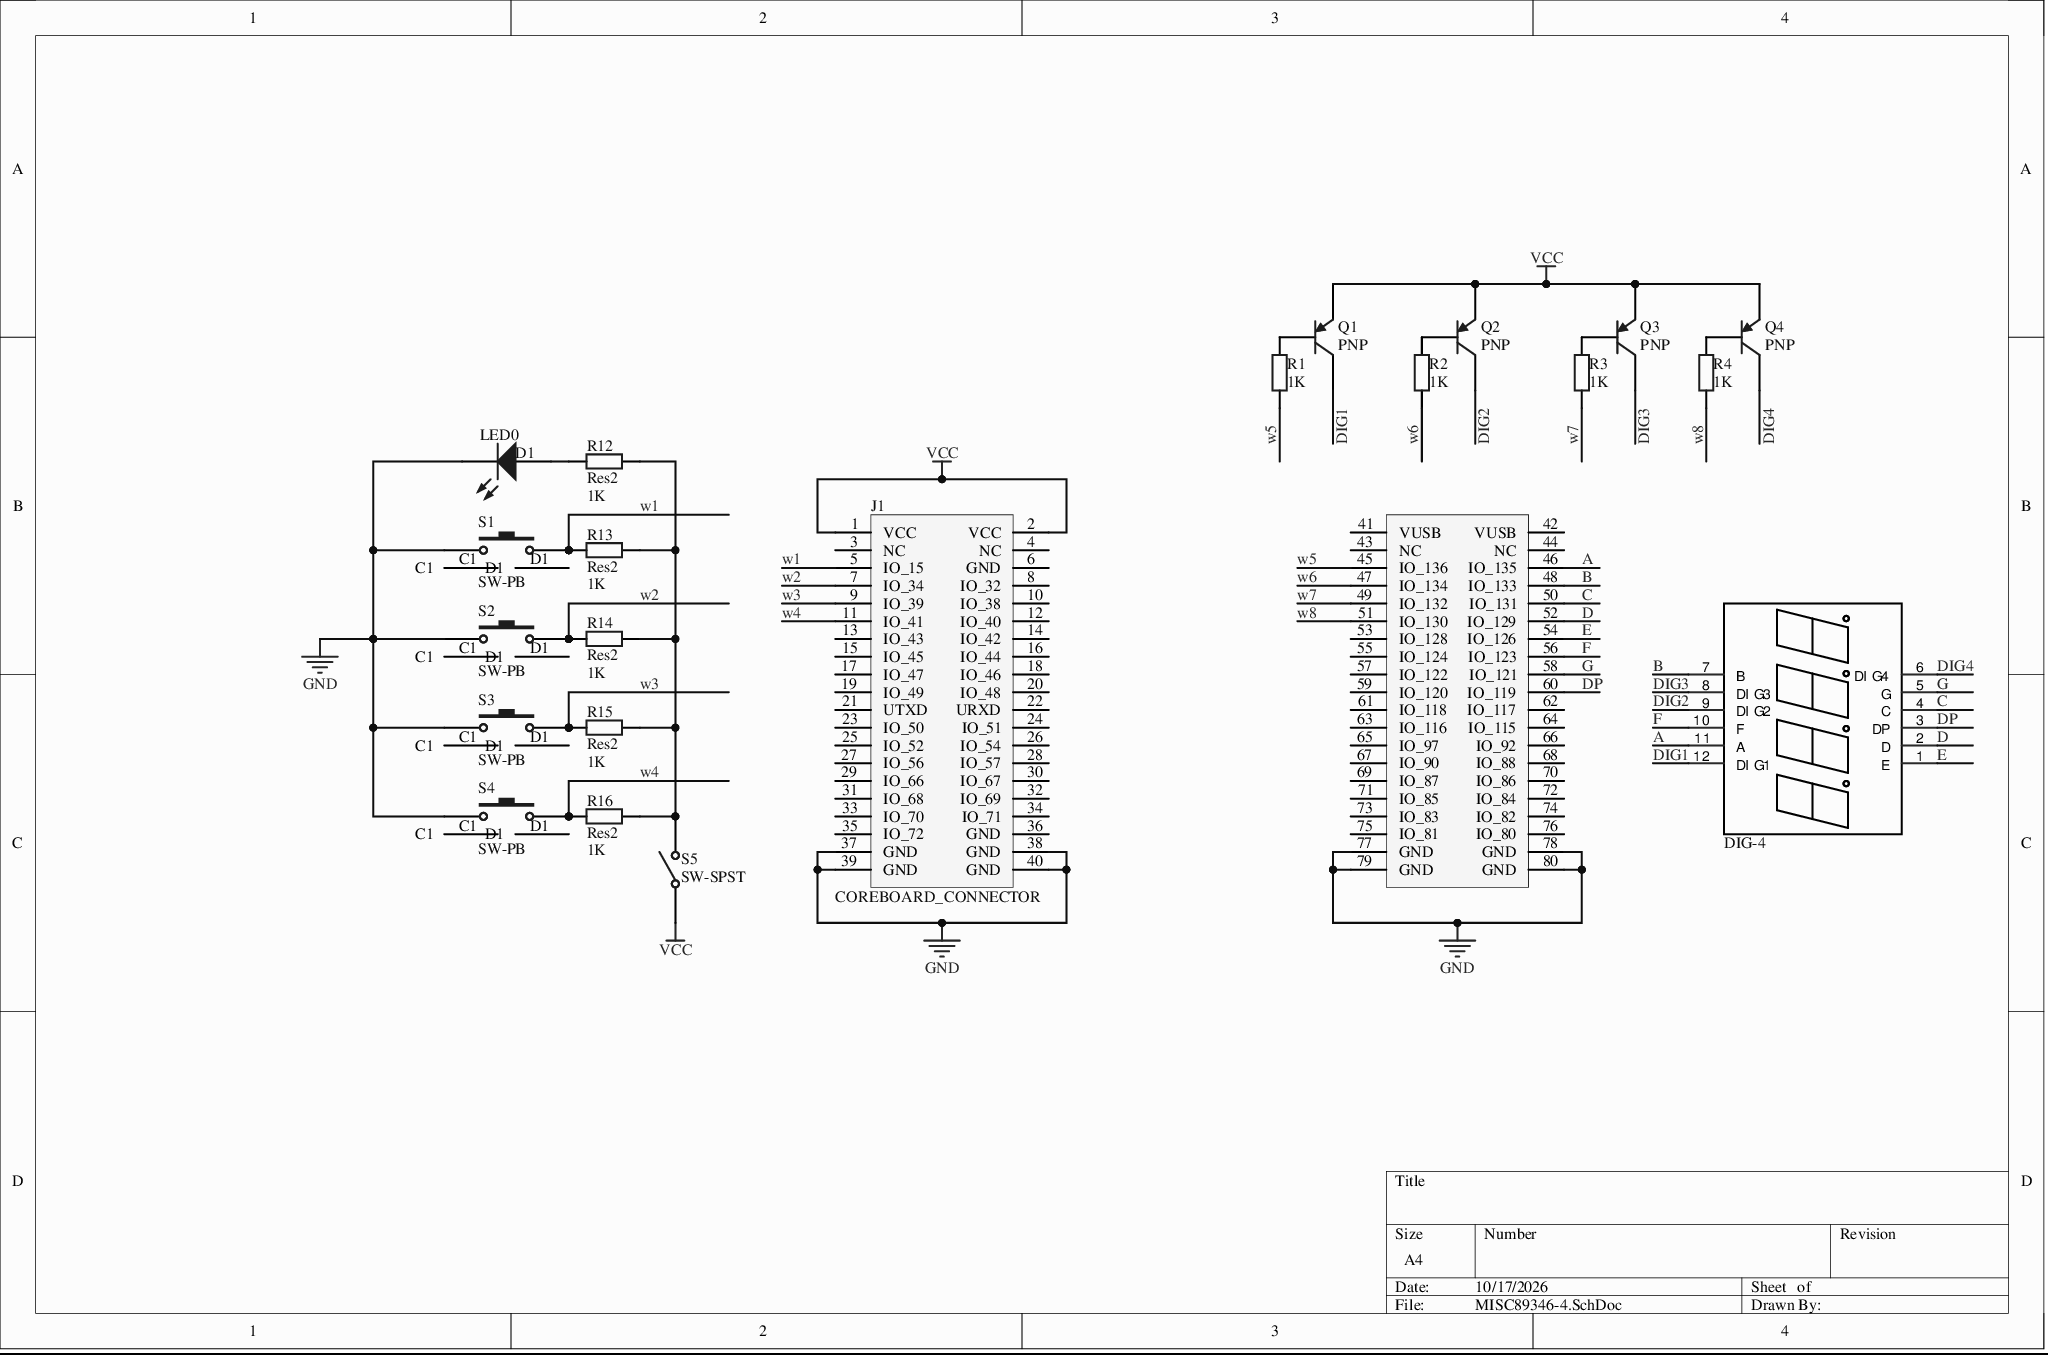
[diagram p0: MISC89346-4.SchDoc]
# Altium project MISC89346-7.PrjPcb
1 sheet, 21 parts. Net scope: global (net labels, ports and power ports of the same name join across sheets).
Board file: MISC89346.PcbDoc

## Sheet MISC89346-4.SchDoc
size A4

### Parts
D1  LED0  [LED_TH_HLMP4700]
J1  COREBOARD_CONNECTOR  [coreboard_connector]
Q1  PNP  [TO-92]
Q2  PNP  [TO-92]
Q3  PNP  [TO-92]
Q4  PNP  [TO-92]
R1  value 1K  [AXIAL-0.5]
R2  value 1K  [AXIAL-0.5]
R3  value 1K  [AXIAL-0.5]
R4  value 1K  [AXIAL-0.5]
R12  Res2  value 1K  [AXIAL-0.5]
R13  Res2  value 1K  [AXIAL-0.5]
R14  Res2  value 1K  [AXIAL-0.5]
R15  Res2  value 1K  [AXIAL-0.5]
R16  Res2  value 1K  [AXIAL-0.5]
S1  SW-PB  [TS665CJ]
S2  SW-PB  [TS665CJ]
S3  SW-PB  [TS665CJ]
S4  SW-PB  [TS665CJ]
S5  SW-SPST  [SS12D10]
  DIG-4  [DIG-4]

### Nets
GND: D1.2(K) J1.37(GND) J1.38(GND) J1.39(GND) J1.40(GND) J1.77(GND) J1.78(GND) J1.79(GND) J1.80(GND) S1.A1(B1) S2.A1(B1) S3.A1(B1) S4.A1(B1)
VCC: J1.1(VCC) J1.2(VCC) Q1.3(E) Q2.3(E) Q3.3(E) Q4.3(E) S5.1(COMMON)
A: J1.46(IO_135) .11(A)
B: J1.48(IO_133) .7(B)
C: J1.50(IO_131) .4(C)
D: J1.52(IO_129) .2(D)
DIG1: .12(DIG1)
DIG2: .9(DIG2)
DIG3: .8(DIG3)
DIG4: .6(DIG4)
DP: J1.60(IO_119) .3(DP)
E: J1.54(IO_126) .1(E)
F: J1.56(IO_123) .10(F)
G: J1.58(IO_121) .5(G)
w1: J1.5(IO_15) R13.1 S1.2
w2: J1.7(IO_34) R14.1 S2.2
w3: J1.9(IO_39) R15.1 S3.2
w4: J1.11(IO_41) R16.1 S4.2
w5: J1.45(IO_136) R1.1
w6: J1.47(IO_134) R2.1
w7: J1.49(IO_132) R3.1
w8: J1.51(IO_130) R4.1
NetD1_1: D1.1(A) R12.1
NetQ1_2: Q1.2(B) R1.2
NetQ2_2: Q2.2(B) R2.2
NetQ3_2: Q3.2(B) R3.2
NetQ4_2: Q4.2(B) R4.2
NetR12_2: R12.2 R13.2 R14.2 R15.2 R16.2 S5.2(NO)

Not connected (* = marked no-connect by the designer): J1 3(NC) 4(NC) 6(GND) 8(IO_32) 10(IO_38) 12(IO_40) 13(IO_43) 14(IO_42) 15(IO_45) 16(IO_44) 17(IO_47) 18(IO_46) 19(IO_49) 20(IO_48) 21(UTXD) 22(URXD) 23(IO_50) 24(IO_51) 25(IO_52) 26(IO_54) 27(IO_56) 28(IO_57) 29(IO_66) 30(IO_67) 31(IO_68) 32(IO_69) 33(IO_70) 34(IO_71) 35(IO_72) 36(GND) 41(VUSB) 42(VUSB) 43(NC) 44(NC) 53(IO_128) 55(IO_124) 57(IO_122) 59(IO_120) 61(IO_118) 62(IO_117) 63(IO_116) 64(IO_115) 65(IO_97) 66(IO_92) 67(IO_90) 68(IO_88) 69(IO_87) 70(IO_86) 71(IO_85) 72(IO_84) 73(IO_83) 74(IO_82) 75(IO_81) 76(IO_80); Q1 1(C); Q2 1(C); Q3 1(C); Q4 1(C); S1 C1 D1; S2 C1 D1; S3 C1 D1; S4 C1 D1

### Notes on the sheet
- Labels drawn without touching a wire or pin: DIG1, DIG2, DIG3, DIG4

### Library data of the parts
D1 = LED0: Typical INFRARED GaAs LED; Published: 8-Jun-2000; LatestRevisionDate: 08-Jul-2005; LatestRevisionNote: Mech Layer 1 removed.; PackageReference: LED-0; PackageDescription: LED; 2 Leads; Publisher: Altium Limited
Q1-Q4 = PNP: PNP Bipolar Transistor; Published: 8-Jun-2000; LatestRevisionDate: 29-May-2009; LatestRevisionNote: IPC-7351 Footprint Added.; PackageVersion: Aug-1999; PackageReference: SOT-23B; PackageDescription: 3-Pin SOT-23 Package 0.95 mm Pitch, 2.4 mm Lead Span; Publisher: Altium Limited
R1-R4 R12-R16 = Res2: Resistor; Published: 8-Jun-2000; LatestRevisionDate: 17-Jul-2002; LatestRevisionNote: Re-released for DXP Platform.; PackageReference: AXIAL-0.4; PackageDescription: Axial Device, Thru-Hole; 2 Leads; 0.4 in Pin Spacing; Publisher: Altium Limited
S1-S4 = SW-PB: Switch; Published: 24-Mar-1999; LatestRevisionDate: 17-Jul-2002; LatestRevisionNote: Re-released for DXP Platform.; PackageReference: SPST-2; PackageDescription: Switch; 2 Leads; Publisher: Altium Limited
S5 = SW-SPST: Single-Pole, Single-Throw Switch; Published: 24-Mar-1999; LatestRevisionDate: 17-Jul-2002; LatestRevisionNote: Re-released for DXP Platform.; PackageReference: SPST-2; PackageDescription: Switch; 2 Leads; Publisher: Altium Limited